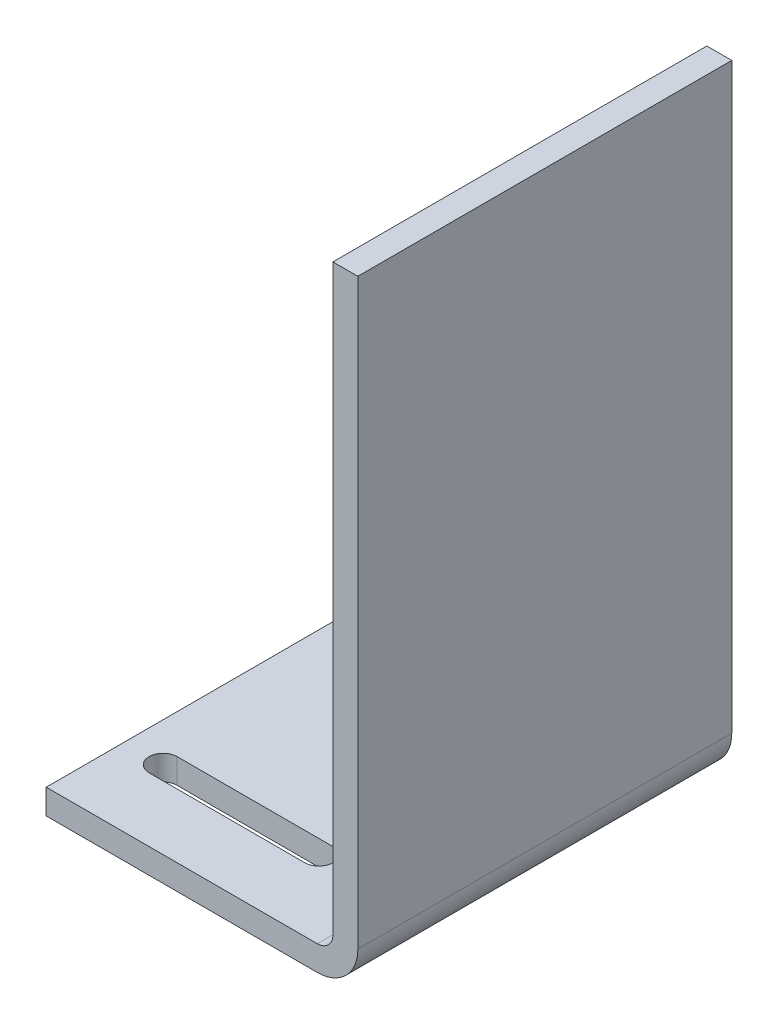
SolidWorks part; units mm, degrees
material "1023 Carbon steel plate (SS)"
ref_plane "Front Plane" through (0, 0, 0) normal (0, 0, 1) x (1, 0, 0)
ref_plane "Top Plane" through (0, 0, 0) normal (0, 1, 0) x (1, 0, 0)
ref_plane "Right Plane" through (0, 0, 0) normal (1, 0, 0) x (0, 0, -1)
sketch "Sketch1" plane through (0, 0, 0) normal (0, 0, 1) x (1, 0, 0)
  line L0 (0, 0) -> (87, 0)
  line L1 (100, 13) -> (100, 200)
  line L2 (0, 8) -> (87, 8)
  line L3 (92, 13) -> (92, 200)
  line L4 (100, 200) -> (92, 200)
  line L5 (0, 8) -> (0, 0)
  arc A0 (87, 0) -> (100, 13) centre (87, 13) ccw
  arc A1 (87, 8) -> (92, 13) centre (87, 13) ccw
  point P6 (100, 0)
  dimension "D3" = 13
  dimension "D1" = 100
  dimension "D2" = 200
  dimension "D4" = 8
extrude "Boss-Extrude1" add sketch "Sketch1" along normal blind 120 contours L5 L0 A0 L1 L4 L3 A1 L2
sketch "Sketch2" plane through (0, 8, 0) normal (0, 1, 0) x (1, 0, 0)
  line L0 (12.5, -25) -> (62.5, -25) construction
  line L1 (12.5, -20.5) -> (62.5, -20.5)
  line L2 (12.5, -29.5) -> (62.5, -29.5)
  line L3 (0, -60) -> (35.7518, -60) construction
  line L4 (0, -120) -> (0, 0) construction
  line L5 (0, 0) -> (87, 0) construction
  line L6 (12.5, -95) -> (62.5, -95) construction
  line L7 (12.5, -99.5) -> (62.5, -99.5)
  line L8 (12.5, -90.5) -> (62.5, -90.5)
  arc A0 (12.5, -20.5) -> (12.5, -29.5) centre (12.5, -25) ccw
  arc A1 (62.5, -29.5) -> (62.5, -20.5) centre (62.5, -25) ccw
  arc A2 (12.5, -99.5) -> (12.5, -90.5) centre (12.5, -95) cw
  arc A3 (62.5, -90.5) -> (62.5, -99.5) centre (62.5, -95) cw
  point P2 (37.5, -25)
  point P15 (37.5, -95)
  dimension "D1" = 9
  dimension "D2" = 50
  dimension "D3" = 20.5
  dimension "D4" = 12.5
extrude "Cut-Extrude1" cut sketch "Sketch2" against normal blind 120
